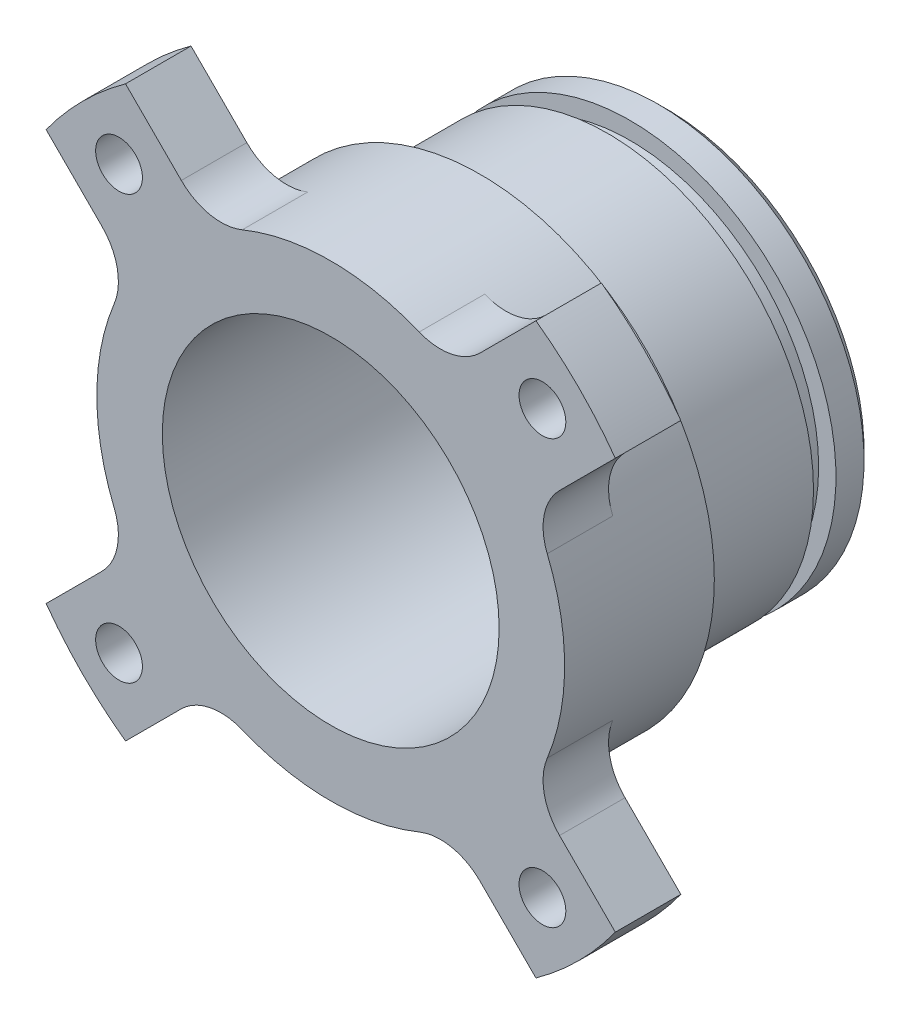
from build123d import *
from build123d.topology import SkipClean

# Parameters (mm, degrees)
SKETCH_1_R          = 11
SKETCH_1_R_2        = 9
EXTRUDE_1_DEPTH     = 6.8
SKETCH_2_R          = 12.5
SKETCH_2_R_2        = 9
EXTRUDE_2_DEPTH     = 8
SKETCH_4_R          = 12.5
SKETCH_4_R_2        = 9
EXTRUDE_3_DEPTH     = 5
CUT_EXTRUDE_START   = -5
SKETCH_8_R          = 12.5
SKETCH_8_R_2        = 9
CUT_EXTRUDE_1_DEPTH = 5
EXTRUDE_START       = -3.5
EXTRUDE_4_DEPTH     = 3.5
HOLE_WIZARD_M3_1_D  = 2.5
FILLET_1_R          = 3
EXTRUDE_START_2     = 1.2
SKETCH_13_R         = 10.075
SKETCH_13_R_2       = 9
EXTRUDE_5_DEPTH     = 1.2
EXTRUDE_START_3     = 2
SKETCH_14_R         = 11
SKETCH_14_R_2       = 9
EXTRUDE_6_DEPTH     = 2
CHAMFER_2_SIZE      = 0.5


with BuildPart() as part:
    # 草图1 → 凸台-拉伸1 (new body)
    with BuildSketch(Plane.XY):
        Circle(SKETCH_1_R)
        Circle(SKETCH_1_R_2, mode=Mode.SUBTRACT)
    extrude(amount=EXTRUDE_1_DEPTH)

    # 草图2 → 凸台-拉伸2 (add)
    with BuildSketch(Plane.XY.offset(6.8)):
        Circle(SKETCH_2_R)
        Circle(SKETCH_2_R_2, mode=Mode.SUBTRACT)
    extrude(amount=EXTRUDE_2_DEPTH)

    # 草图4 → 凸台-拉伸3 (add)
    with BuildSketch(Plane.XY.offset(14.8)):
        Circle(SKETCH_4_R)
        Circle(SKETCH_4_R_2, mode=Mode.SUBTRACT)
    extrude(amount=EXTRUDE_3_DEPTH)

    # 草图8 → 切除-拉伸1 (cut)
    with BuildSketch(Plane.XY.offset(19.8).offset(CUT_EXTRUDE_START)):
        Circle(SKETCH_8_R)
        Circle(SKETCH_8_R_2, mode=Mode.SUBTRACT)
    extrude(amount=CUT_EXTRUDE_1_DEPTH, mode=Mode.SUBTRACT)

    # 草图9 → 凸台-拉伸4 (add)
    with BuildSketch(Plane.XY.offset(14.8).offset(EXTRUDE_START)):
        with BuildLine():
            Line((10.966125931, 15.208766619), (6.459180807, 10.701821494))
            ThreePointArc((6.459180807, 10.701821494), (8.838834765, 8.838834765), (10.701821494, 6.459180807))
            Line((10.701821494, 6.459180807), (15.208766619, 10.966125931))
            ThreePointArc((15.208766619, 10.966125931), (13.258252147, 13.258252147), (10.966125931, 15.208766619))
        make_face()
        with BuildLine():
            Line((15.208766619, -10.966125931), (10.701821494, -6.459180807))
            ThreePointArc((10.701821494, -6.459180807), (8.838834765, -8.838834765), (6.459180807, -10.701821494))
            Line((6.459180807, -10.701821494), (10.966125931, -15.208766619))
            ThreePointArc((10.966125931, -15.208766619), (13.258252147, -13.258252147), (15.208766619, -10.966125931))
        make_face()
        with BuildLine():
            Line((-10.966125931, -15.208766619), (-6.459180807, -10.701821494))
            ThreePointArc((-6.459180807, -10.701821494), (-8.838834765, -8.838834765), (-10.701821494, -6.459180807))
            Line((-10.701821494, -6.459180807), (-15.208766619, -10.966125931))
            ThreePointArc((-15.208766619, -10.966125931), (-13.258252147, -13.258252147), (-10.966125931, -15.208766619))
        make_face()
        with BuildLine():
            Line((-15.208766619, 10.966125931), (-10.701821494, 6.459180807))
            ThreePointArc((-10.701821494, 6.459180807), (-8.838834765, 8.838834765), (-6.459180807, 10.701821494))
            Line((-6.459180807, 10.701821494), (-10.966125931, 15.208766619))
            ThreePointArc((-10.966125931, 15.208766619), (-13.258252147, 13.258252147), (-15.208766619, 10.966125931))
        make_face()
    extrude(amount=EXTRUDE_4_DEPTH)

    # M3 螺纹孔1 (through all)
    with Locations(Plane.XY.offset(14.8)):
        with Locations((-11.313708499, 11.313708499), (11.313708499, 11.313708499), (11.313708499, -11.313708499), (-11.313708499, -11.313708499)):
            Hole(HOLE_WIZARD_M3_1_D / 2)

    # 圆角1
    fillet_1_edges = [part.edges().sort_by_distance(p)[0] for p in [
        (10.701821494, 6.459180807, 13.05),
        (6.459180807, 10.701821494, 13.05),
        (6.459180807, -10.701821494, 13.05),
        (10.701821494, -6.459180807, 13.05),
        (-10.701821494, -6.459180807, 13.05),
        (-6.459180807, -10.701821494, 13.05),
        (-6.459180807, 10.701821494, 13.05),
        (-10.701821494, 6.459180807, 13.05),
    ]]
    fillet(fillet_1_edges, radius=FILLET_1_R)

    # 草图13 → 凸台-拉伸5 (add)
    with SkipClean():  # the faces are left unmerged after this step: merging them gives an invalid solid
        with BuildSketch(Plane(origin=(0, 0, 0), x_dir=(-1, 0, 0), z_dir=(0, 0, -1)).offset(EXTRUDE_START_2)):
            with Locations(Location((0, 0, 0), (0, 0, 180))):
                Circle(SKETCH_13_R)
            Circle(SKETCH_13_R_2, mode=Mode.SUBTRACT)
        extrude(amount=-EXTRUDE_5_DEPTH)

    # 草图14 → 凸台-拉伸6 (add)
    with SkipClean():  # the faces are left unmerged after this step: merging them gives an invalid solid
        with BuildSketch(Plane(origin=(0, 0, -1.2), x_dir=(-1, 0, 0), z_dir=(0, 0, -1)).offset(EXTRUDE_START_3)):
            with Locations(Location((0, 0, 0), (0, 0, 180))):
                Circle(SKETCH_14_R)
            Circle(SKETCH_14_R_2, mode=Mode.SUBTRACT)
        extrude(amount=-EXTRUDE_6_DEPTH)

    # 倒角2
    chamfer_2_edges = [part.edges().sort_by_distance(p)[0] for p in [
        (-11, 0, -3.2),
    ]]
    chamfer(chamfer_2_edges, length=CHAMFER_2_SIZE)


solid = part.part
